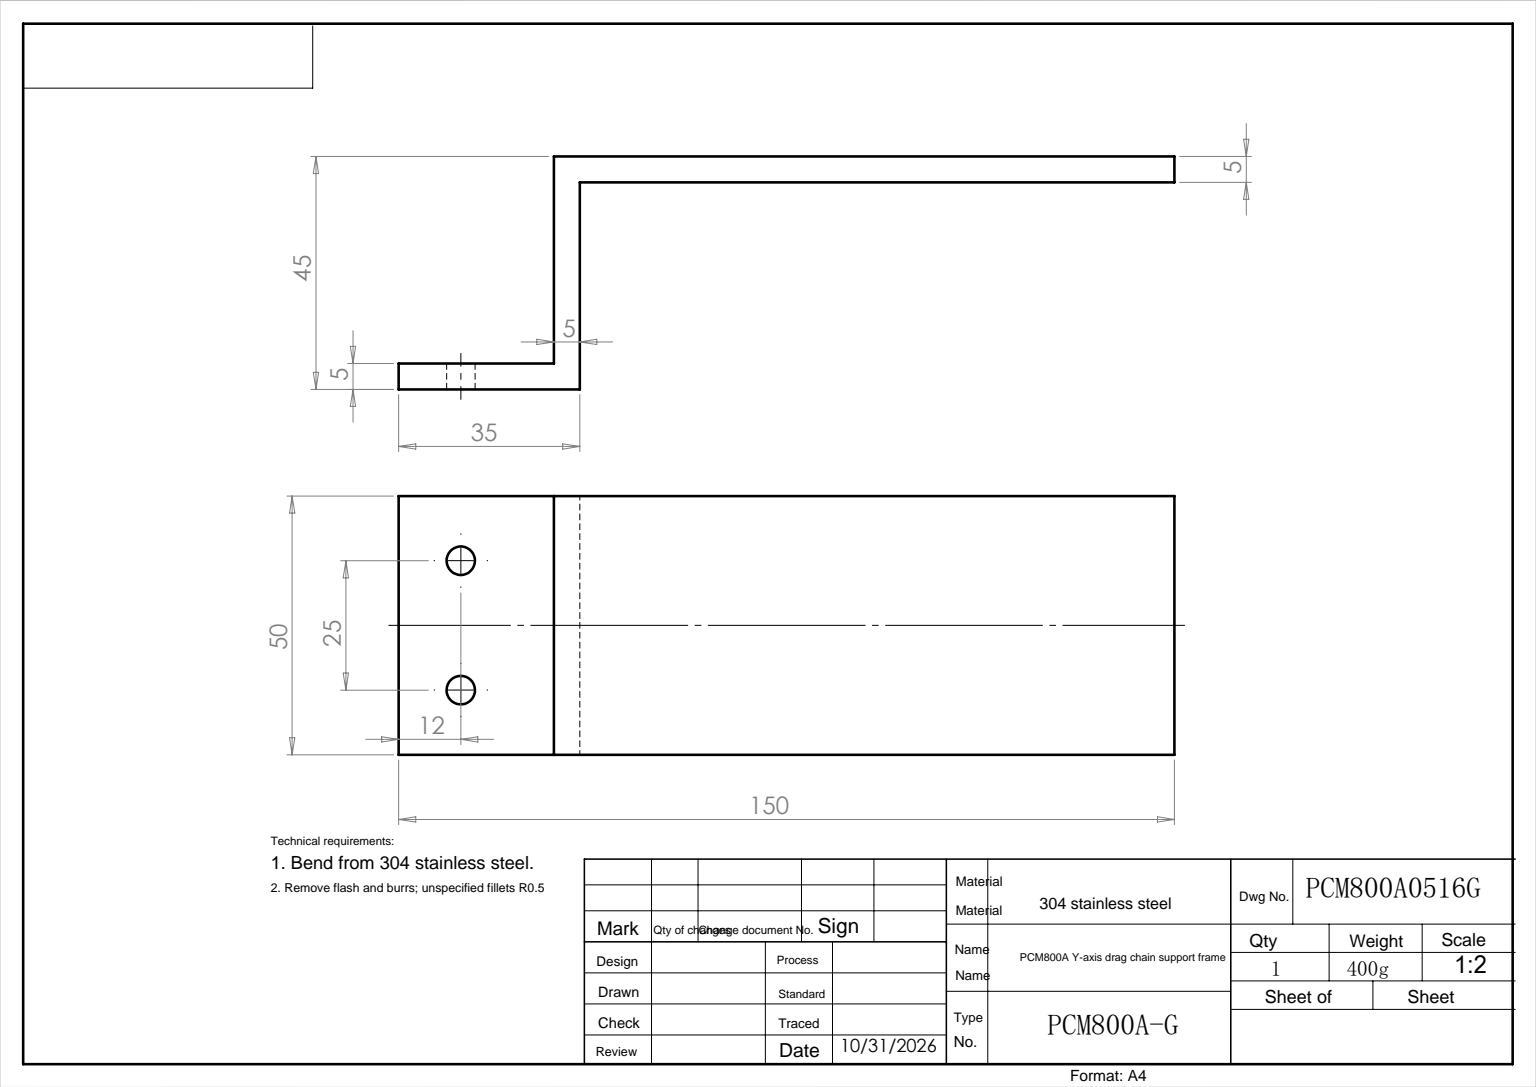
from build123d import *

# Parameters (mm, degrees)
EXTRUDE_1_DEPTH     = 50
SKETCH_2_R          = 2.75
CUT_EXTRUDE_1_DEPTH = 10


with BuildPart() as part:
    # 草图1 → 拉伸-薄壁1 (new body)
    with BuildSketch(Plane.XY):
        Polygon((0, 0), (30, 0), (30, 40), (150, 40), (150, 35), (35, 35), (35, -5), (0, -5), align=None)
    extrude(amount=EXTRUDE_1_DEPTH)

    # 草图2 → 切除-拉伸1 (cut)
    with BuildSketch(Plane(origin=(0, 0, 0), x_dir=(1, 0, 0), z_dir=(0, 1, 0))):
        with Locations(Location((12, -12.5, 0), (0, 0, 270))):
            Circle(SKETCH_2_R)
        with Locations(Location((12, -37.5, 0), (0, 0, 270))):
            Circle(SKETCH_2_R)
    extrude(amount=-CUT_EXTRUDE_1_DEPTH, mode=Mode.SUBTRACT)


solid = part.part
